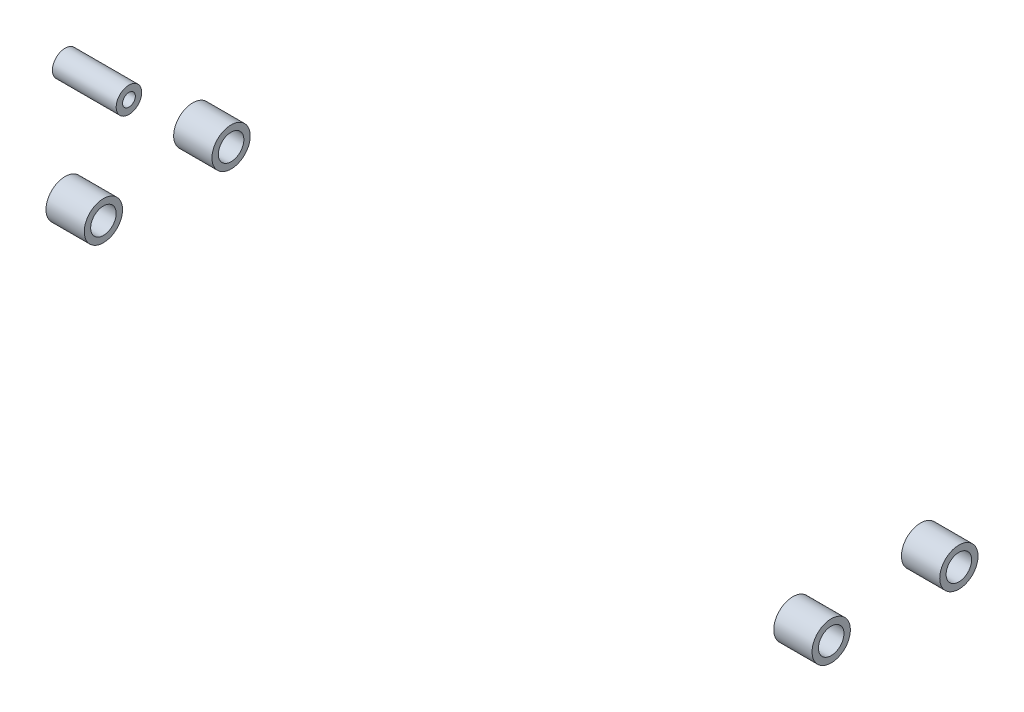
from build123d import *

# Parameters (mm, degrees)
SKETCH1_W           = 30
SKETCH1_H           = 5
SKETCH3_R           = 10
SKETCH3_R_2         = 5
BOSS_EXTRUDE1_DEPTH = 50


with BuildPart() as part:
    # Sketch1 → Revolve1 (revolve)
    with BuildSketch(Plane.XY, mode=Mode.PRIVATE) as revolve1_sk:
        with Locations((-285, 12.5)):
            Rectangle(SKETCH1_W, SKETCH1_H)
        with Locations((285, 12.5)):
            Rectangle(SKETCH1_W, SKETCH1_H)
    revolve(revolve1_sk.sketch.rotate(Axis((-367.380839301, 0, 0), (1, 0, 0)), 90), axis=Axis((-367.380839301, 0, 0), (1, 0, 0)))


with BuildPart() as body_2:
    # Mirror5: mirrored copy
    add(part.part.mirror(Plane.XY.offset(50)))


with BuildPart() as body_3:
    # Sketch3 → Boss-Extrude1 (new body)
    with BuildSketch(Plane.ZY.offset(300)):
        with Locations((50, 42)):
            Circle(SKETCH3_R)
        with Locations((50, 42)):
            Circle(SKETCH3_R_2, mode=Mode.SUBTRACT)
    extrude(amount=BOSS_EXTRUDE1_DEPTH)


solid = Compound([part.part, body_2.part, body_3.part])
